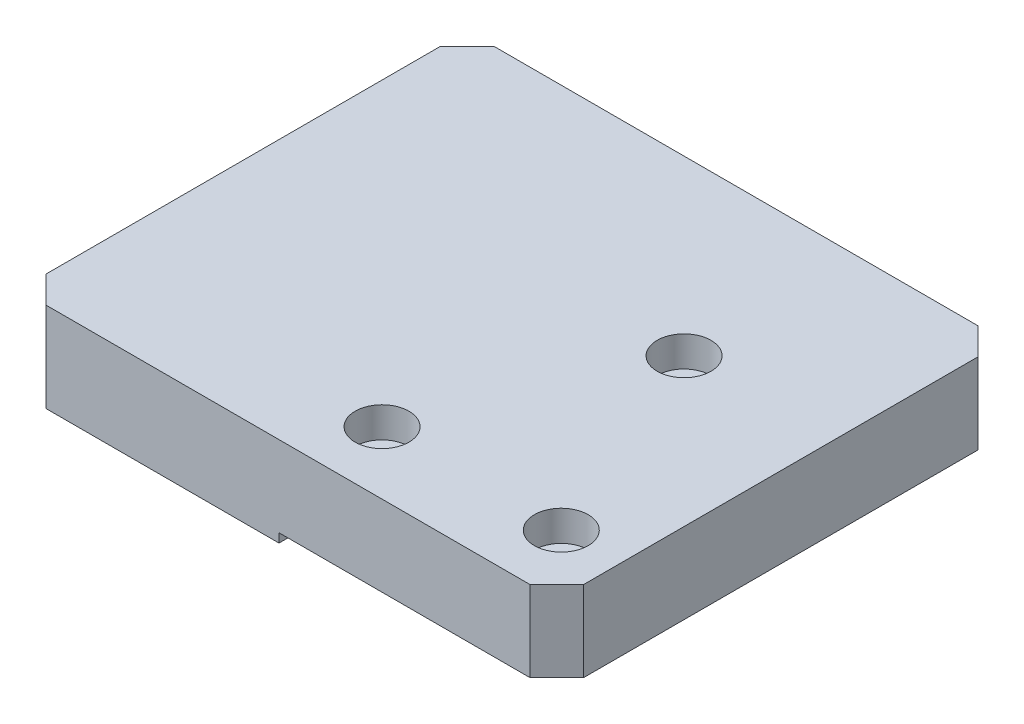
SolidWorks part; units mm, degrees
material "A6061 T6"
ref_plane "前视基准面" through (0, 0, 0) normal (0, 0, 1) x (1, 0, 0)
ref_plane "上视基准面" through (0, 0, 0) normal (0, 1, 0) x (1, 0, 0)
ref_plane "右视基准面" through (0, 0, 0) normal (1, 0, 0) x (0, 0, -1)
sketch "草图1" plane through (0, 0, 0) normal (0, 1, 0) x (1, 0, 0)
  line L1 (-30, 25) -> (30, 25)
  line L2 (-30, 25) -> (-30, -25)
  line L3 (-30, -25) -> (30, -25)
  line L4 (30, 25) -> (30, -25)
  line L5 (-30, 25) -> (30, -25) construction
  line L6 (-30, -25) -> (30, 25) construction
  point P0 (0, 0)
  dimension "D1" = 60
  dimension "D2" = 50
extrude "凸台-拉伸1" add sketch "草图1" along normal blind 10
sketch "草图5" plane through (0, 0, 0) normal (0, -1, 0) x (1, 0, 0)
  line L0 (-30, 25) -> (30, 25) construction
  line L1 (-1, 25) -> (30, 25)
  line L2 (-1, 25) -> (-1, -25)
  line L3 (-1, -25) -> (30, -25)
  line L4 (30, 25) -> (30, -25)
  line L5 (30, -25) -> (-30, -25) construction
  line L6 (30, 25) -> (30, -25) construction
  dimension "D1" = 31
extrude "切除-拉伸1" cut sketch "草图5" against normal blind 1
chamfer "倒角2" distance 3 angle 45 4 edges at (-30, 5, -25) (-30, 5, 25) (30, 5.5, -25) (30, 5.5, 25)
hole_wizard "M5 螺纹孔1" positions "草图14" profile "草图15" tap size "M5" standard "GB"
sketch "草图14" plane through (-30, 0, 0) normal (-1, 0, 0) x (0, 0, 1)
  line L0 (-22, 0) -> (22, 0) construction
  line L1 (25, 10) -> (25, 0) construction
  line L2 (-25, 0) -> (-25, 10) construction
  point P0 (17, 5)
  point P2 (-17, 4.9743)
  point P4 (0, 4.9743)
  dimension "D1" = 5
  dimension "D2" = 8
  dimension "D3" = 8
  dimension "D4" = 17
sketch "草图15" plane through (-30, 5, 17) normal (0, 1, 0) x (0, 0, 1)
  line L0 (0, 0) -> (0, 13.6618)
  line L1 (0, 13.6618) -> (2.1, 12.4)
  line L2 (2.1, 12.4) -> (2.1, 0)
  line L5 (2.1, 0) -> (0, 0)
  line L10 (0, 13.6618) -> (-2.1, 12.4) construction
  line L11 (0, -6.35) -> (0, 107.95) construction
  dimension "螺纹孔钻头直径" = 4.2
  dimension "螺纹孔钻头深度" = 12.4
  dimension "导头角度" = 118
cosmetic thread "孔螺蚊线1"
cosmetic thread "孔螺蚊线2"
cosmetic thread "孔螺蚊线3"
hole_wizard "打孔尺寸(%根据)内六角圆柱头螺钉的类型3" positions "草图16" profile "草图17" counterbore size "M3" standard "GB"
sketch "草图16" plane through (0, 10, 0) normal (0, 1, 0) x (1, 0, 0)
  point P0 (23.5, -18)
  point P3 (3.5, -18)
  point P6 (13.5, 5.7)
sketch "草图17" plane through (23.5, 10, 18) normal (1, 0, 0) x (0, 0, 1)
  line L0 (0, 0) -> (0, 13.4215)
  line L1 (0, 13.4215) -> (1.7, 12.4)
  line L2 (1.7, 12.4) -> (1.7, 3.4)
  line L3 (1.7, 3.4) -> (3, 3.4)
  line L4 (3, 3.4) -> (3, 0)
  line L5 (3, 0) -> (0, 0)
  line L10 (0, 13.4215) -> (-1.7, 12.4) construction
  line L11 (0, -6.35) -> (0, 107.95) construction
  dimension "孔直径" = 3.4
  dimension "孔深度" = 12.4
  dimension "柱形沉头孔直径" = 6
  dimension "柱形沉头孔深度" = 3.4
  dimension "导头角度" = 118
hole_wizard "大小mm 暗销孔3" positions "草图18" profile "草图19" hole size "Ø4.0" standard "GB"
sketch "草图18" plane through (-30, 0, 0) normal (-1, 0, 0) x (0, 0, 1)
  line L0 (-22, 10) -> (22, 10) construction
  line L1 (25, 10) -> (25, 0) construction
  line L2 (-25, 0) -> (-25, 10) construction
  point P0 (9, 5)
  point P2 (-9, 5)
  dimension "D1" = 5
  dimension "D2" = 16
  dimension "D3" = 16
sketch "草图19" plane through (-30, 5, 9) normal (0, 1, 0) x (0, 0, 1)
  line L0 (0, 0) -> (0, 13.6017)
  line L1 (0, 13.6017) -> (2, 12.4)
  line L2 (2, 12.4) -> (2, 0)
  line L5 (2, 0) -> (0, 0)
  line L10 (0, 13.6017) -> (-2, 12.4) construction
  line L11 (0, -6.35) -> (0, 107.95) construction
  dimension "孔直径" = 4
  dimension "孔深度" = 12.4
  dimension "导头角度" = 118
